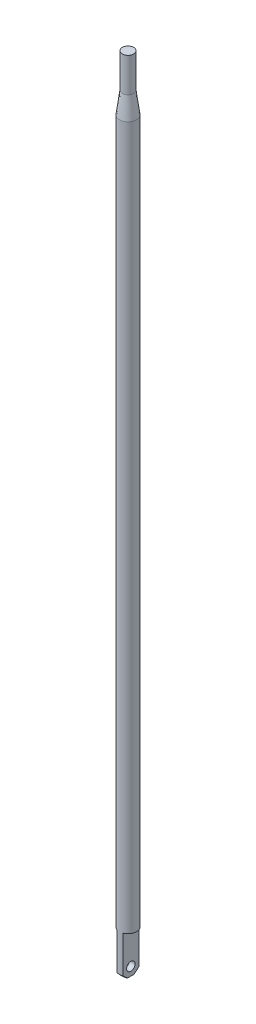
from build123d import *

# Parameters (mm, degrees)
CUT_EXTRUDE1_DEPTH      = 562.064167453
CUT_EXTRUDE1_DEPTH_BACK = 562.064167453
SKETCH2_W               = 4
SKETCH2_H               = 29
CUT_EXTRUDE2_DEPTH      = 562.064167453
CUT_EXTRUDE2_DEPTH_BACK = 562.064167453
SKETCH3_W               = 4
SKETCH3_H               = 29
CHAMFER1_SIZE           = 3
SKETCH4_R               = 3
CUT_EXTRUDE3_DEPTH      = 4


with BuildPart() as part:
    # Sketch1 → Revolve1 (revolve)
    with BuildSketch(Plane.XY):
        Polygon((0, 561), (4, 561), (4, 537), (6, 522), (6, 0), (0, 0), align=None)
    revolve(axis=Axis((0, -719.526877718, 0), (0, 1, 0)))

    # Sketch2 → Cut-Extrude1 (cut, two sides: drawn at the far end of the back side and taken through both)
    with BuildSketch(Plane.XY.offset(-CUT_EXTRUDE1_DEPTH_BACK)):
        with Locations((-4, 14.5)):
            Rectangle(SKETCH2_W, SKETCH2_H)
    extrude(amount=CUT_EXTRUDE1_DEPTH + CUT_EXTRUDE1_DEPTH_BACK, mode=Mode.SUBTRACT)

    # Sketch3 → Cut-Extrude2 (cut, two sides: drawn at the far end of the back side and taken through both)
    with BuildSketch(Plane.XY.offset(-CUT_EXTRUDE2_DEPTH_BACK)):
        with Locations((4, 14.5)):
            Rectangle(SKETCH3_W, SKETCH3_H)
    extrude(amount=CUT_EXTRUDE2_DEPTH + CUT_EXTRUDE2_DEPTH_BACK, mode=Mode.SUBTRACT)

    # Chamfer1
    chamfer1_edges = [part.edges().sort_by_distance(p)[0] for p in [
        (0, 0, -6),
        (0, 0, 6),
    ]]
    chamfer(chamfer1_edges, length=CHAMFER1_SIZE)

    # Sketch4 → Cut-Extrude3 (cut)
    with BuildSketch(Plane.ZY.offset(2)):
        with Locations((0, 6)):
            Circle(SKETCH4_R)
    extrude(amount=-CUT_EXTRUDE3_DEPTH, mode=Mode.SUBTRACT)


solid = part.part
